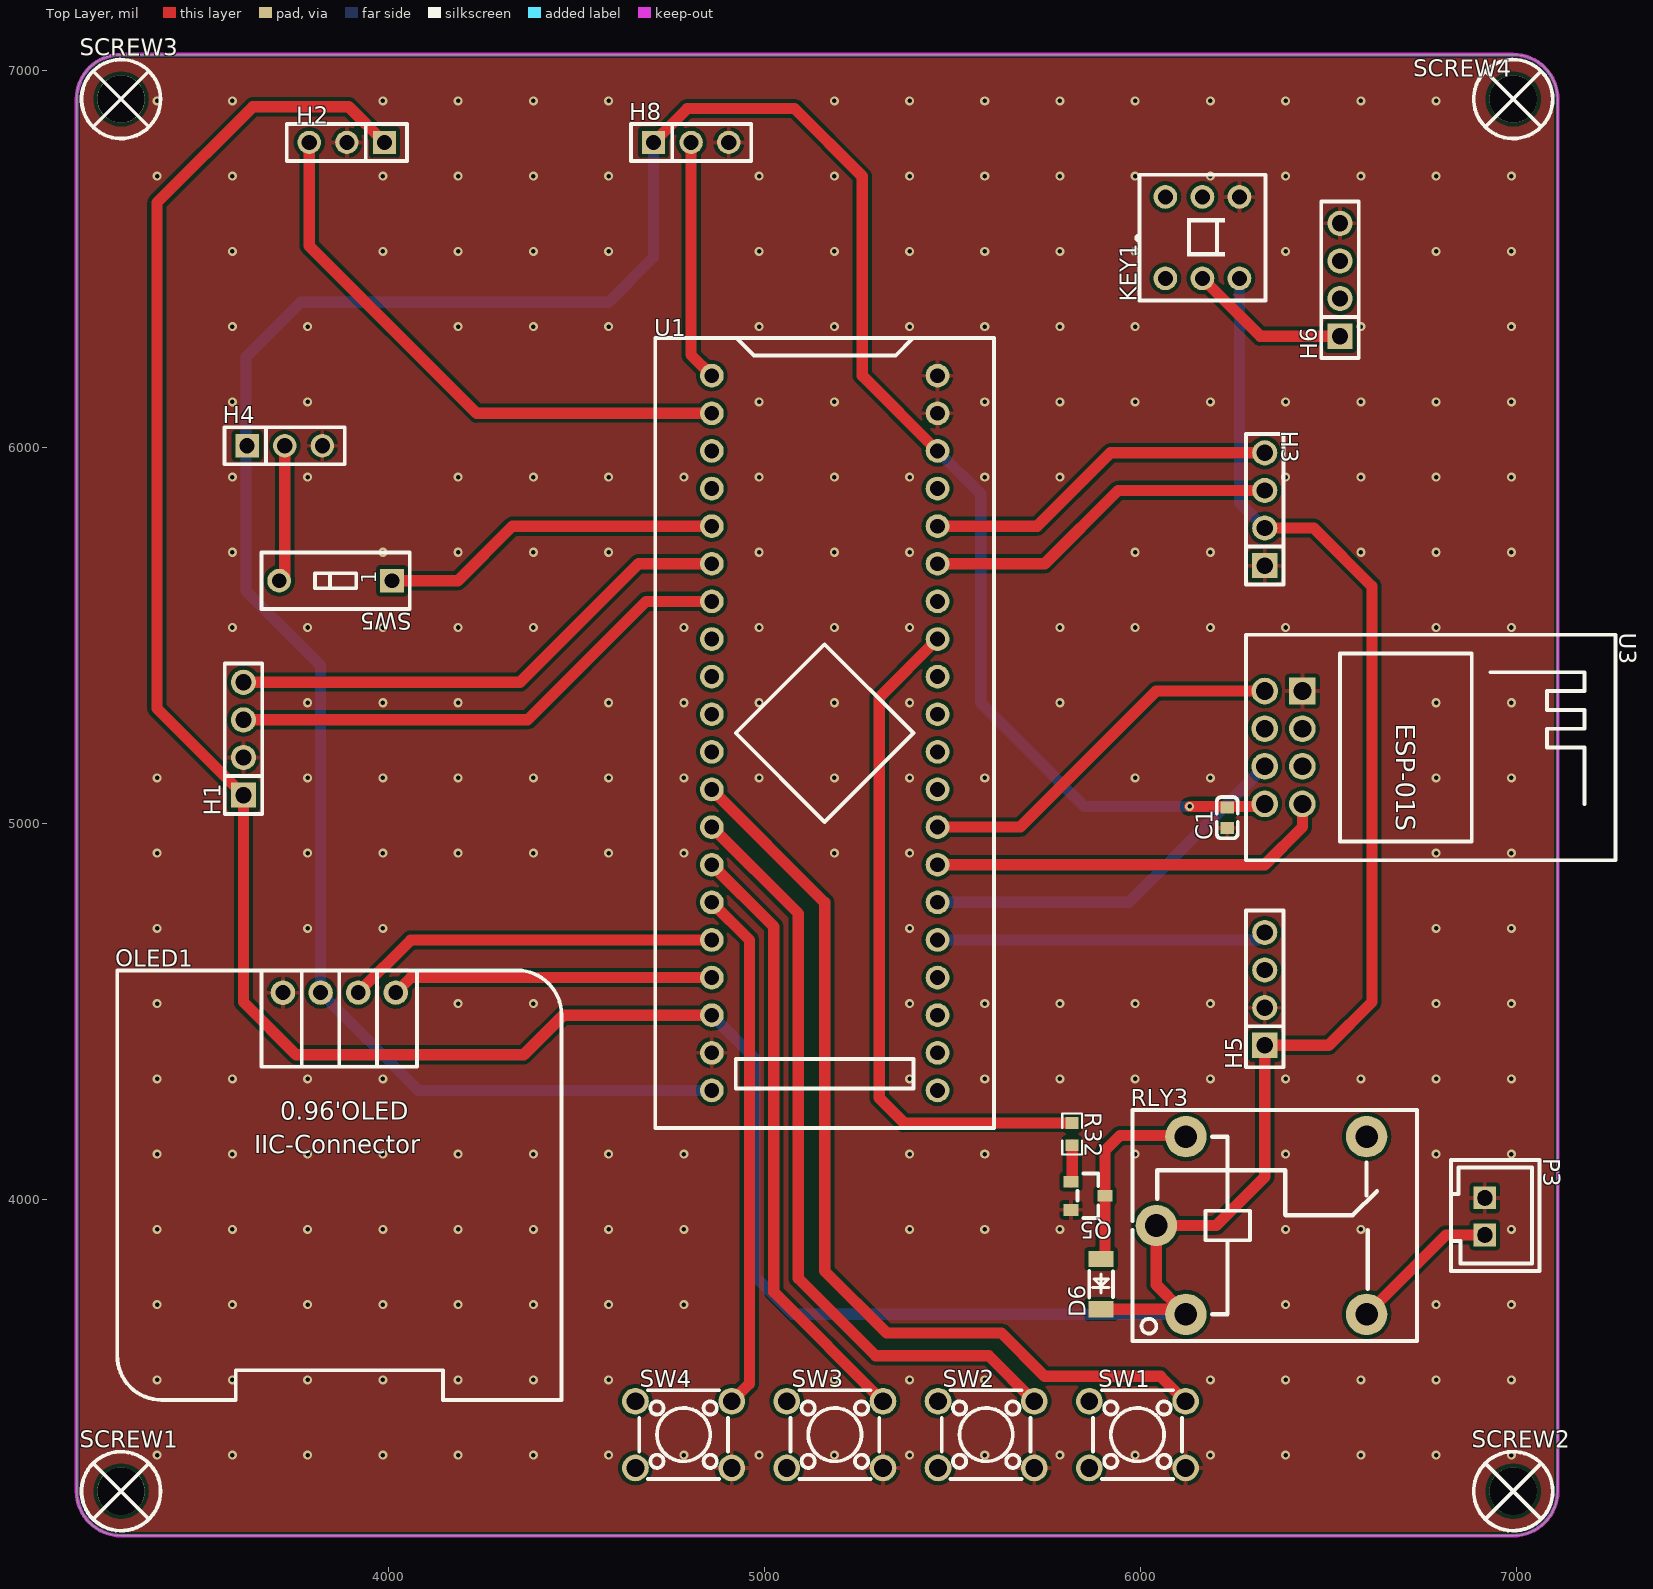
[diagram p0: Top Layer view]
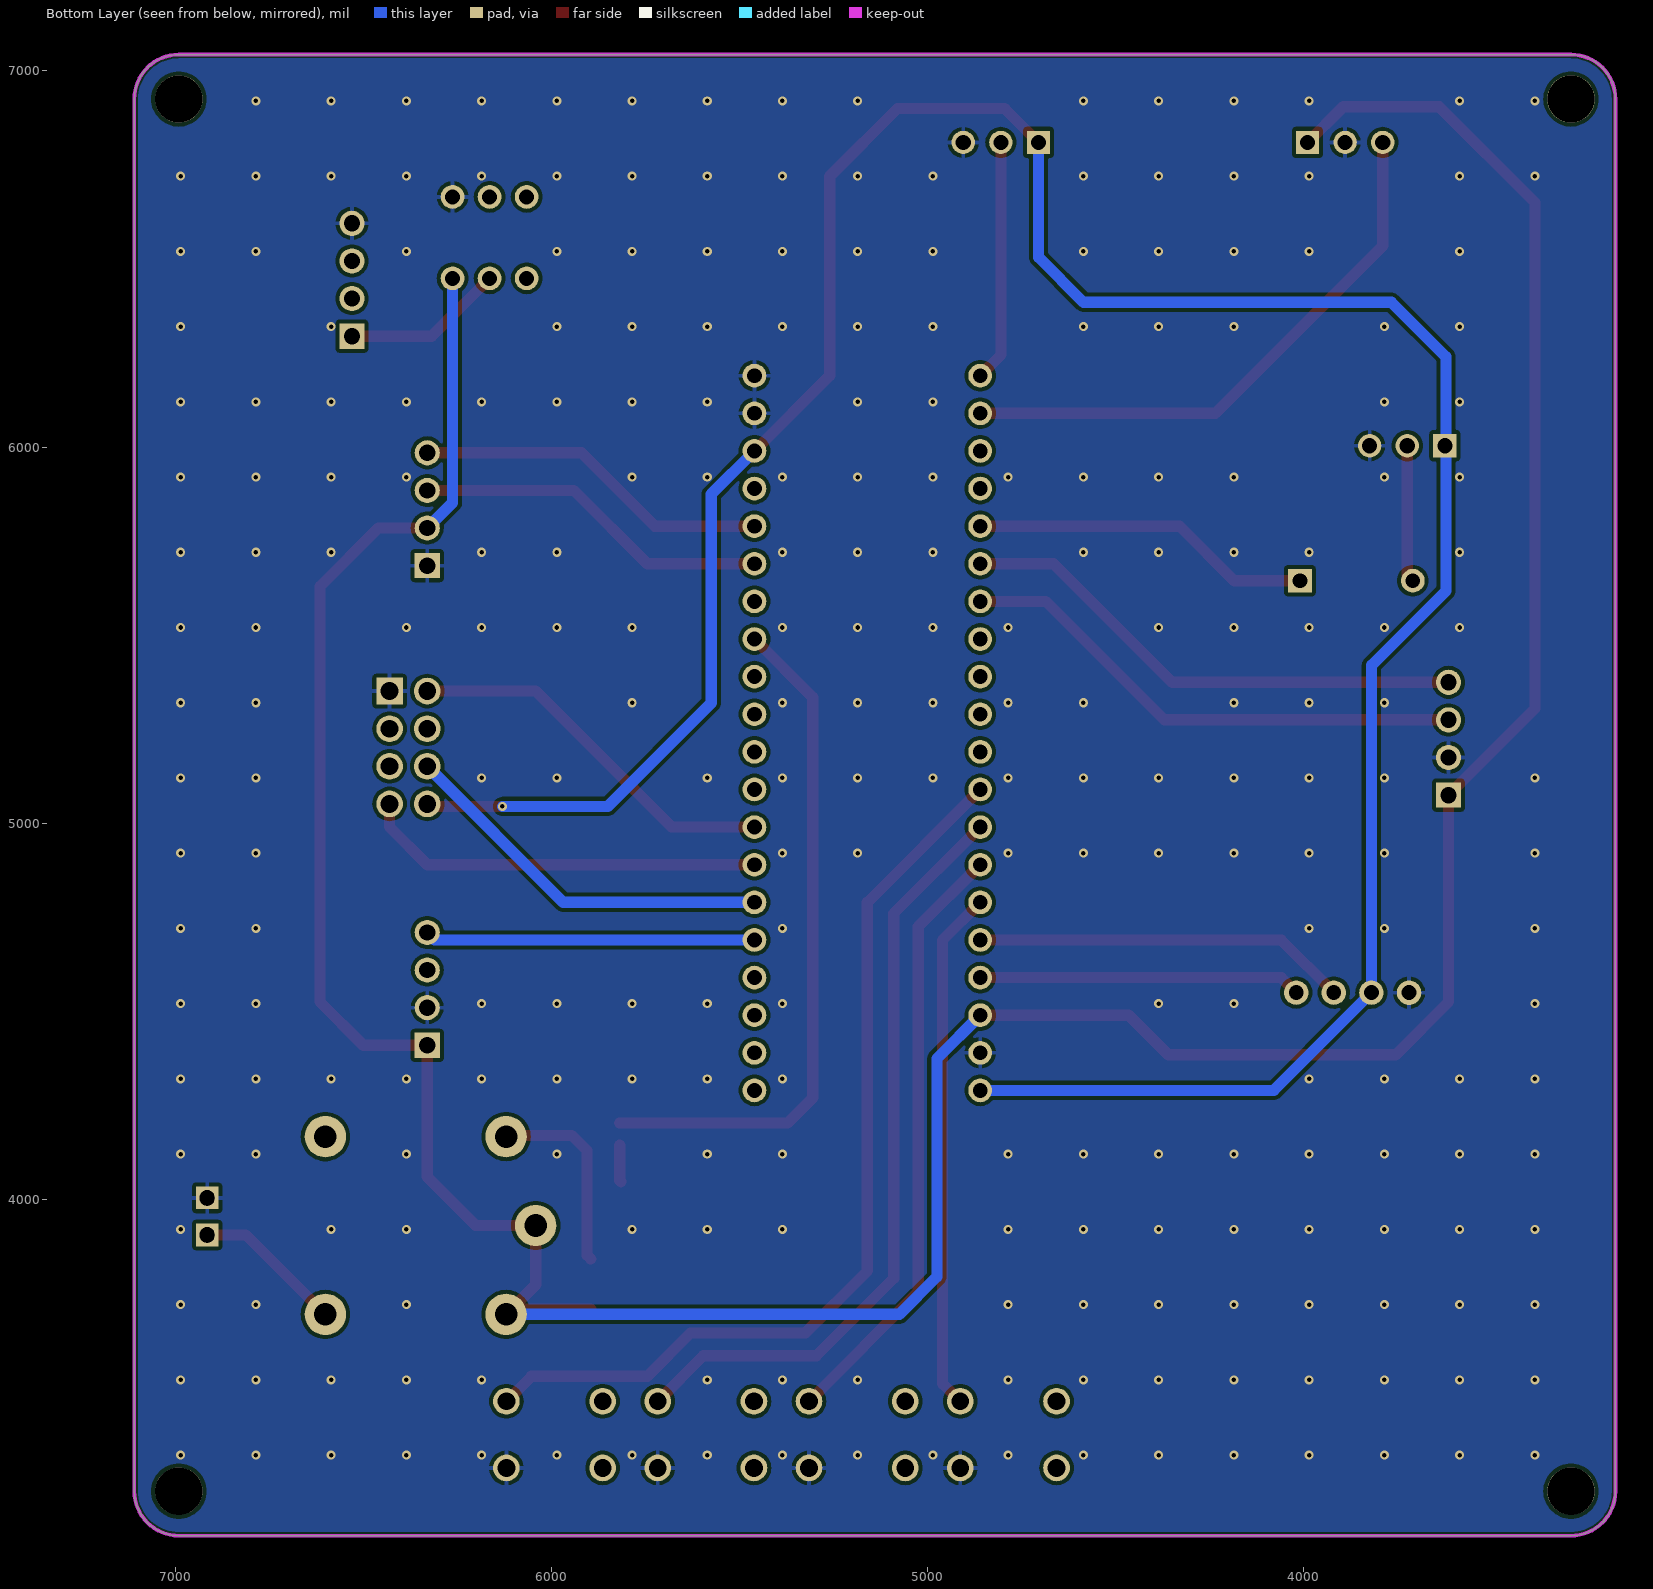
[diagram p1: Bottom Layer view, seen from below]
# Altium PCB MISC75114.pcbdoc
Units mil, origin at the board's own origin, x right, y up, seen from the top; angles counter-clockwise.
Board outline 3937.01 x 3937.01 mil, 2 copper layers (Top Layer, Bottom Layer), stack 62.206 mil thick; 26 components, 42 nets, 121 pads, 255 vias.

## Layer stack, top to bottom
Top Solder Mask Layer: solder mask 0.394, Dk 3.3
Top Layer: signal copper 1.379
Dielectric1: surface 59.449, FR4, Dk 4.5
Bottom Layer: signal copper 1.378
Bottom Solder Mask Layer: solder mask 0.394, Dk 3.3

## Board outline
6990.39,3106.5 ccw(c6990.39,3224.61) 7108.5,3224.61 7108.5,6925.39 ccw(c6990.39,6925.39) 6990.39,7043.5 3289.61,7043.5 ccw(c3289.61,6925.39) 3171.5,6925.39 3171.5,3224.61 ccw(c3289.61,3224.61) 3289.61,3106.5

## Design rules (kind name [scope] priority, off if disabled: settings)
BoardOutlineClearance copperThickness2oz_1 [All] p2 off: genericclearance=7.99 ignorepadtopadclearanceinfootprint=FALSE except(0: Arc-SplitContinuation Track-SplitContinuation SMDPad-SplitContinuation THPad-SplitContinuation Via-SplitContinuation Fill-SplitContinuation Region-SplitContinuation Poly-SplitContinuation Text-SplitContinuation Hole-SplitContinuation; 5.98: Arc-CutoutEdge Track-CutoutEdge SMDPad-CutoutEdge THPad-CutoutEdge Via-CutoutEdge Text-CutoutEdge; 6.89: Hole-OutlineEdge Hole-CutoutEdge; 10: Poly-OutlineEdge Poly-CutoutEdge; 11.81: Arc-OutlineEdge Track-OutlineEdge SMDPad-OutlineEdge THPad-OutlineEdge Via-OutlineEdge Fill-OutlineEdge Region-OutlineEdge Text-OutlineEdge Fill-CutoutEdge Region-CutoutEdge)
BoardOutlineClearance Plane_innerPlane_1 [All] p4 off: genericclearance=4.02 ignorepadtopadclearanceinfootprint=FALSE except(0: Arc-SplitContinuation Track-SplitContinuation SMDPad-SplitContinuation THPad-SplitContinuation Via-SplitContinuation Fill-SplitContinuation Region-SplitContinuation Poly-SplitContinuation Text-SplitContinuation Hole-SplitContinuation; 5.98: Arc-CutoutEdge Track-CutoutEdge SMDPad-CutoutEdge THPad-CutoutEdge Via-CutoutEdge Text-CutoutEdge; 6.89: Hole-OutlineEdge Hole-CutoutEdge; 10: Poly-OutlineEdge Poly-CutoutEdge; 11.81: Arc-OutlineEdge Track-OutlineEdge SMDPad-OutlineEdge THPad-OutlineEdge Via-OutlineEdge Fill-OutlineEdge Region-OutlineEdge Text-OutlineEdge Fill-CutoutEdge Region-CutoutEdge)
BoardOutlineClearance Copper_copperRegion_1 [All] p6 off: genericclearance=4.02 ignorepadtopadclearanceinfootprint=FALSE except(0: Arc-SplitContinuation Track-SplitContinuation SMDPad-SplitContinuation THPad-SplitContinuation Via-SplitContinuation Fill-SplitContinuation Region-SplitContinuation Poly-SplitContinuation Text-SplitContinuation Hole-SplitContinuation; 5.98: Arc-CutoutEdge Track-CutoutEdge SMDPad-CutoutEdge THPad-CutoutEdge Via-CutoutEdge Text-CutoutEdge; 6.89: Hole-OutlineEdge Hole-CutoutEdge; 10: Poly-OutlineEdge Poly-CutoutEdge; 11.81: Arc-OutlineEdge Track-OutlineEdge SMDPad-OutlineEdge THPad-OutlineEdge Via-OutlineEdge Fill-OutlineEdge Region-OutlineEdge Text-OutlineEdge Fill-CutoutEdge Region-CutoutEdge)
BoardOutlineClearance copperThickness1oz_1 [All] p8: genericclearance=4.02 ignorepadtopadclearanceinfootprint=FALSE except(0: Arc-SplitContinuation Track-SplitContinuation SMDPad-SplitContinuation THPad-SplitContinuation Via-SplitContinuation Fill-SplitContinuation Region-SplitContinuation Poly-SplitContinuation Text-SplitContinuation Hole-SplitContinuation; 5.98: Arc-CutoutEdge Track-CutoutEdge SMDPad-CutoutEdge THPad-CutoutEdge Via-CutoutEdge Text-CutoutEdge; 6.89: Hole-OutlineEdge Hole-CutoutEdge; 10: Poly-OutlineEdge Poly-CutoutEdge; 11.81: Arc-OutlineEdge Track-OutlineEdge SMDPad-OutlineEdge THPad-OutlineEdge Via-OutlineEdge Fill-OutlineEdge Region-OutlineEdge Text-OutlineEdge Fill-CutoutEdge Region-CutoutEdge)
Clearance copperThickness2oz [All] p1 off: gap=7.99 ignorepadtopadclearanceinfootprint=FALSE except(5.98: SMDPad-Track SMDPad-SMDPad THPad-Track SMDPad-THPad THPad-THPad Track-Via SMDPad-Via THPad-Via Via-Via Fill-SMDPad Region-SMDPad Fill-THPad Region-THPad Fill-Via Region-Via Fill-Fill Fill-Region Region-Region Arc-Track Arc-SMDPad Arc-THPad Arc-Via Fill-Arc Region-Arc Arc-Arc Text-Track SMDPad-Text Text-THPad Text-Via Fill-Text Region-Text Arc-Text Text-Text; 6.89: Hole-Track Hole-SMDPad Hole-THPad Hole-Via Fill-Hole Region-Hole Hole-Arc Hole-Text; 10: Poly-Track Poly-SMDPad Poly-THPad Poly-Via Poly-Fill Poly-Region Poly-Poly Poly-Arc Poly-Text Poly-Hole; 11.81: Fill-Track Region-Track)
Clearance Plane_innerPlane [All] p3 off: gap=4.02 ignorepadtopadclearanceinfootprint=FALSE except(5.98: SMDPad-Track SMDPad-SMDPad THPad-Track SMDPad-THPad THPad-THPad Track-Via SMDPad-Via THPad-Via Via-Via Fill-SMDPad Region-SMDPad Fill-THPad Region-THPad Fill-Via Region-Via Fill-Fill Fill-Region Region-Region Arc-Track Arc-SMDPad Arc-THPad Arc-Via Fill-Arc Region-Arc Arc-Arc Text-Track SMDPad-Text Text-THPad Text-Via Fill-Text Region-Text Arc-Text Text-Text; 6.89: Hole-Track Hole-SMDPad Hole-THPad Hole-Via Fill-Hole Region-Hole Hole-Arc Hole-Text; 10: Poly-Track Poly-SMDPad Poly-THPad Poly-Via Poly-Fill Poly-Region Poly-Poly Poly-Arc Poly-Text Poly-Hole; 11.81: Fill-Track Region-Track)
Clearance Copper_copperRegion [All] p5 off: gap=4.02 ignorepadtopadclearanceinfootprint=FALSE except(5.98: SMDPad-Track SMDPad-SMDPad THPad-Track SMDPad-THPad THPad-THPad Track-Via SMDPad-Via THPad-Via Via-Via Fill-SMDPad Region-SMDPad Fill-THPad Region-THPad Fill-Via Region-Via Fill-Fill Fill-Region Region-Region Arc-Track Arc-SMDPad Arc-THPad Arc-Via Fill-Arc Region-Arc Arc-Arc Text-Track SMDPad-Text Text-THPad Text-Via Fill-Text Region-Text Arc-Text Text-Text; 6.89: Hole-Track Hole-SMDPad Hole-THPad Hole-Via Fill-Hole Region-Hole Hole-Arc Hole-Text; 10: Poly-Track Poly-SMDPad Poly-THPad Poly-Via Poly-Fill Poly-Region Poly-Poly Poly-Arc Poly-Text Poly-Hole; 11.81: Fill-Track Region-Track)
Clearance copperThickness1oz [All] p7: gap=4.02 ignorepadtopadclearanceinfootprint=FALSE except(5.98: SMDPad-Track SMDPad-SMDPad THPad-Track SMDPad-THPad THPad-THPad Track-Via SMDPad-Via THPad-Via Via-Via Fill-SMDPad Region-SMDPad Fill-THPad Region-THPad Fill-Via Region-Via Fill-Fill Fill-Region Region-Region Arc-Track Arc-SMDPad Arc-THPad Arc-Via Fill-Arc Region-Arc Arc-Arc Text-Track SMDPad-Text Text-THPad Text-Via Fill-Text Region-Text Arc-Text Text-Text; 6.89: Hole-Track Hole-SMDPad Hole-THPad Hole-Via Fill-Hole Region-Hole Hole-Arc Hole-Text; 10: Poly-Track Poly-SMDPad Poly-THPad Poly-Via Poly-Fill Poly-Region Poly-Poly Poly-Arc Poly-Text Poly-Hole; 11.81: Fill-Track Region-Track)
DiffPairsRouting differentialPair [All] p1: maxlimit=6 minlimit=6 mostfreqgap=6 toplayer_minwidth=5 toplayer_prefwidth=10 toplayer_maxwidth=100 toplayer_mingap=6 toplayer_prefgap=6 toplayer_maxgap=6 bottomlayer_minwidth=5 bottomlayer_prefwidth=10 bottomlayer_maxwidth=100 bottomlayer_mingap=6 bottomlayer_prefgap=6 bottomlayer_maxgap=6 maxuncoupledlength=10
HoleToHoleClearance otherClearance [All] p1: gap=11.81 allowstackedmicrovias=TRUE
Length netLength [All] p1: minlimit=0 maxlimit=0
PasteMaskExpansion pasteMaskExpansion [All] p1: expansion=0
PlaneConnect innerPlane [All] p1: planeconnectstyle=Relief reliefexpansion=20 reliefentries=4 reliefconductorwidth=10 reliefairgap=10
PolygonConnect copperRegion [All] p1: connectstyle=Relief reliefconductorwidth=10 reliefentries=4 polygonreliefangle="90 Angle" airgapwidth=10 via.connectstyle=Relief via.reliefconductorwidth=10 via.reliefentries=4 via.polygonreliefangle="90 Angle" via.airgapwidth=10
RoutingVias viaSize [All] p1: holewidth=12.01 width=24.02 viastyle="Through Hole" minholewidth=11.81 minwidth=19.68 maxholewidth=248.03 maxwidth=393.7
SolderMaskExpansion solderMaskExpansion [IsVia] p1: expansion=-1000 istentingtop=TRUE
SolderMaskExpansion solderMaskExpansion [All] p2: expansion=2.01 istentingtop=FALSE
Width copperThickness2oz_2 [All] p1 off: maxlimit=100 minlimit=8 preferedwidth=10
Width copperThickness1oz_2 [All] p2: maxlimit=100 minlimit=5 preferedwidth=30

## Components (designator, comment, footprint, x,y, rotation, side; value= is the part's Value field where it differs from the comment)
C1 "1uF" C0603 6230,5015 r90 top
D6 "LL4148" LL-34_L3.5-W1.5-RD 5895,3775 r90 top
H1 "" HDR-TH_4P-P2.54-V-M 3615,5225 r90 top
H2 "" HDR-TH_3P-P2.54-V-F 3890,6810 r180 top
H3 "" HDR-TH_4P-P2.54-V-M 6329.9,5835 r90 top
H4 "" HDR-TH_3P-P2.54-V-F 3724.74,6003.84 r0 top
H5 "" HDR-TH_4P-P2.54-V-F 6329.9,4560 r90 top
H6 "" HDR-TH_4P-P2.54-V-F 6530,6445 r90 top
H8 "" HDR-TH_3P-P2.54-V-F 4805,6810 r0 top
KEY1 "Non-latching switch 8.5×8.5 silent" SW-TH_6P-L8.5-W8.5-P2.54 6164.22,6556.9 r0 top
OLED1 "" 0.96OLED_4P 3870,4550 r0 top
P3 "XH2.54 through-hole socket-2P" CONN-TH_XH2.54-2P 6915,3954.99 r270 top
Q5 "" S8050_SOT-23 5860,4015 r180 top
R32 "1k" R0603 5817.82,4173.92 r270 top
RLY3 "SRD-05VDC-SL-C" RELAY-TH_SRD-XXVDC-XL-C 6321.15,3930.95 r0 top
SCREW1 "" M3螺丝 3289.61,3224.61 r0 top
SCREW2 "" M3螺丝 6990.39,3224.61 r0 top
SCREW3 "" M3螺丝 3289.61,6925.39 r0 top
SCREW4 "" M3螺丝 6990.39,6925.39 r0 top
SW1 "" SW-TH_4P-L6.0-W6.0-P4.50-LS6.5 5991.57,3375 r180 top
SW2 "" SW-TH_4P-L6.0-W6.0-P4.50-LS6.5 5589.38,3375 r180 top
SW3 "" SW-TH_4P-L6.0-W6.0-P4.50-LS6.5 5187.19,3375 r180 top
SW4 "" SW-TH_4P-L6.0-W6.0-P4.50-LS6.5 4785,3375 r180 top
SW5 "NDS-01V" SW-TH_2P-L3.9-W9.9-P2.54-LS7.6 3860,5645 r180 top
U1 "STM32F103C8T6-Card" CONN-TH_L53.3-W22.9_STM32F103C8T6-CARD 5160,5240 r270 top
U3 "ESP-01S" WIFIM-TH_ESP-01S 6380,5201.63 r270 top

## Footprints (in the part's own frame and the unit in brackets; to place one, negate y for a bottom-side part, rotate by r counter-clockwise, add the part's x,y. Pads: shape width x height; smd on the part's side, far side on the other; paste and mask are expansions set on the pad)
0.96OLED_4P [mm]
  round 1.65 hole 1 copper offset 0,0: 1(-3.81,-0.001) 2(-1.27,0.002) 3(1.27,0.002) 4(3.81,0.002)
  silkscreen extent -15,-27.5 15,1.5
C0603 [mm]
  rect 0.8x0.9 smd: 1(-0.7,0) 2(0.7,0)
  silkscreen extent -1.39,-0.71 1.39,0.71
CONN-TH_L53.3-W22.9_STM32F103C8T6-CARD [mm]
  round 1.6 hole 1: 1(-24.13,-7.62) 2(-21.59,-7.62) 3(-19.05,-7.62) 4(-16.51,-7.62) 5(-13.97,-7.62) 6(-11.43,-7.62) 7(-8.89,-7.62) 8(-6.35,-7.62) 9(-3.81,-7.62) 10(-1.27,-7.62) 11(1.27,-7.62) 12(3.81,-7.62) 13(6.35,-7.62) 14(8.89,-7.62) 15(11.43,-7.62) 16(13.97,-7.62) 17(16.51,-7.62) 18(19.05,-7.62) 19(21.59,-7.62) 20(24.13,-7.62) 21(24.13,7.62) 22(21.59,7.62) 23(19.05,7.62) 24(16.51,7.62) 25(13.97,7.62) 26(11.43,7.62) 27(8.89,7.62) 28(6.35,7.62) 29(3.81,7.62) 30(1.27,7.62) 31(-1.27,7.62) 32(-3.81,7.62) 33(-6.35,7.62) 34(-8.89,7.62) 35(-11.43,7.62) 36(-13.97,7.62) 37(-16.51,7.62) 38(-19.05,7.62) 39(-21.59,7.62) 40(-24.13,7.62)
  silkscreen extent -26.67,-11.43 26.67,11.43
CONN-TH_XH2.54-2P [mil]
  rect 60x60 hole 39.37 slot 41.34 at 0 deg paste+0 mask+1.97: 1(-49.22,0) 2(49.21,0)
  silkscreen extent -150,-90 145,145
HDR-TH_3P-P2.54-V-F [mil]
  rect 62x62 hole 40.16: 1(-100,0)
  round 62 hole 40.16: 2(0,0) 3(100,0)
  silkscreen extent -160,-49 160,49
HDR-TH_4P-P2.54-V-F [mm]
  rect 1.7x1.7 hole 1.1: 1(-3.81,0)
  round 1.7 hole 1.1: 2(-1.27,0) 3(1.27,0) 4(3.81,0)
  silkscreen extent -5.29,-1.27 5.29,1.27
HDR-TH_4P-P2.54-V-M [mm]
  rect 1.7x1.7 hole 1.1: 1(-3.81,0)
  round 1.7 hole 1.1: 2(-1.27,0) 3(1.27,0) 4(3.81,0)
  silkscreen extent -5.08,-1.27 5.08,1.27
LL-34_L3.5-W1.5-RD [mm]
  rect 1.1x1.7 smd paste+0 mask+0.051: 1(-1.7,0) 2(1.7,0)
  silkscreen extent -0.9,-0.8 0.9,0.8
M3螺丝 [mil]
  round 126 hole 126 paste+0 mask+4: 1(0,0)
  silkscreen extent -105,-105 105,105
R0603 [mil]
  rect 31.75x34.02 smd paste-3937.01 mask+2: 1(-29.66,0) 2(29.66,0)
  silkscreen extent -55,-26 55,26
RELAY-TH_SRD-XXVDC-XL-C [mil]
  round 110 hole 60: 1(-200.79,-236.22) 2(279.52,-236.2) 3(279.53,236.2) 4(-200.79,236.22) 5(-279.53,0)
  silkscreen extent -342,-307 413,307
S8050_SOT-23 [mm]
  rect 1x0.8 smd paste+0 mask+0.051: 1(1.15,-0.823) 2(1.15,1.077) 3(-1.15,0.127)
  silkscreen extent -0.7,-1.37 0.7,1.63
SW-TH_2P-L3.9-W9.9-P2.54-LS7.6 [mm]
  rect 1.6x1.6 hole 1 paste+0 mask+0.05: 1(-3.81,0)
  round 1.6 hole 1 paste+0 mask+0.05: 2(3.81,0)
  silkscreen extent -5,-1.91 5,1.91
SW-TH_4P-L6.0-W6.0-P4.50-LS6.5 [mm]
  round 1.8 hole 1.2: 1(-3.25,2.25) 2(3.25,2.25) 3(-3.25,-2.25) 4(3.25,-2.25)
  silkscreen extent -3,-3 3,3
SW-TH_6P-L8.5-W8.5-P2.54 [mm]
  round 1.6 hole 1: 1(-2.5,-2.75) 2(0,-2.75) 3(2.5,-2.75) 4(-2.5,2.75) 5(0,2.75) 6(2.5,2.75)
  silkscreen extent -4.47,-4.25 4.25,4.25
WIFIM-TH_ESP-01S [mm]
  rect 1.8x1.8 hole 1.2: 1(-3.81,1.27)
  round 1.8 hole 1.2: 2(-1.27,1.27) 3(1.27,1.27) 4(3.81,1.27) 5(3.81,-1.27) 6(1.27,-1.27) 7(-1.27,-1.27) 8(-3.81,-1.27)
  silkscreen extent -7.62,-2.54 7.62,22.4

## Via types
v1: diameter 24.02, hole 12, Top Layer to Bottom Layer, 255 vias

## Nets (pads, with @x,y where several pads share a name; then routed paths per layer and width w, separated by ;. In a path a pad name is that pad's centre, name@x,y a point inside that pad or via, vN(x,y) a via of type N, cw(c..) or ccw(c..) an arc to the next point about the centre after c; other vN are vias at no path point)
$1N18282: H6.1 KEY1.2 | length 429.4
  Top Layer w30: KEY1.2 6317.84,6295 H6.1
$1N18356: Q5.1 R32.2 | length 98.1
  Top Layer w30: Q5.1 5817.82,4050.5 R32.2
$1N18358: D6.2 Q5.3 RLY3.4 | length 525.3
  Top Layer w30: D6.2 5905.28,3852.21 Q5.3 5905.28,4130.28 5945,4170 6117.53,4170 RLY3.4
$1N18360: P3.2 RLY3.2 | length 401.7
  Top Layer w30: RLY3.2 6811.7,3905.78 P3.2
$1N18374: H4.2 SW5.2 | length 364.9
  Top Layer w30: SW5.2 3724.74,5659.74 H4.2
+5V: D6.1 H1.1 H2.1 H3.2 H5.1 KEY1.3 RLY3.1 RLY3.5 U1.18 | length 9878.6
  Top Layer w30: H2.1 3895,6905 3640,6905 3385,6650 3385,5305 H1.1 3615,4525 3755,4385 4360,4385 4465,4490 U1.18 ; D6.1 6107.02,3708.07 6041.62,3773.47 RLY3.5 6200.95,3930.95 6329.9,4059.9 H5.1 6500,4410 6615,4525 6615,5630 6460,5785 H3.2
  Bottom Layer w30: U1.18 4975,4375 4975,3795 5075.27,3694.73 RLY3.1 ; KEY1.3 6262.64,5852.26 H3.2
GND: C1.1 H1.2 H2.2 H3.1 H4.3 H5.2 H6.4 H8.3 KEY1.6 OLED1.1 P3.1 Q5.2 SW1.1 SW2.1 SW3.1 SW4.1 U1.19 U1.39 U1.40 U3.1
  other v1: 3385.6,3320.6 3585.6,3320.6 3785.6,3320.6 3985.6,3320.6 4185.6,3320.6 4385.6,3320.6 4585.6,3320.6 4785.6,3320.6 4985.6,3320.6 5185.6,3320.6 5385.6,3320.6 5585.6,3320.6 5785.6,3320.6 5985.6,3320.6 6185.6,3320.6 6385.6,3320.6 6585.6,3320.6 6785.6,3320.6 6985.6,3320.6 3385.6,3520.6 3585.6,3520.6 3785.6,3520.6 3985.6,3520.6 4185.6,3520.6 4385.6,3520.6 4585.6,3520.6 4785.6,3520.6 5185.6,3520.6 5385.6,3520.6 5585.6,3520.6 6185.6,3520.6 6385.6,3520.6 6585.6,3520.6 6785.6,3520.6 6985.6,3520.6 3385.6,3720.6 3585.6,3720.6 3785.6,3720.6 3985.6,3720.6 4185.6,3720.6 4385.6,3720.6 4585.6,3720.6 4785.6,3720.6 6385.6,3720.6 6785.6,3720.6 6985.6,3720.6 3385.6,3920.6 3585.6,3920.6 3785.6,3920.6 3985.6,3920.6 4185.6,3920.6 4385.6,3920.6 4585.6,3920.6 4785.6,3920.6 5385.6,3920.6 5585.6,3920.6 5785.6,3920.6 6385.6,3920.6 6585.6,3920.6 6985.6,3920.6 3385.6,4120.6 3585.6,4120.6 3785.6,4120.6 3985.6,4120.6 4185.6,4120.6 4385.6,4120.6 4585.6,4120.6 4785.6,4120.6 5385.6,4120.6 5585.6,4120.6 5985.6,4120.6 6385.6,4120.6 6785.6,4120.6 6985.6,4120.6 3385.6,4320.6 3585.6,4320.6 3785.6,4320.6 3985.6,4320.6 5385.6,4320.6 5585.6,4320.6 5785.6,4320.6 5985.6,4320.6 6185.6,4320.6 6385.6,4320.6 6585.6,4320.6 6785.6,4320.6 6985.6,4320.6 3385.6,4520.6 4185.6,4520.6 4385.6,4520.6 5385.6,4520.6 5585.6,4520.6 5785.6,4520.6 5985.6,4520.6 6185.6,4520.6 6785.6,4520.6 6985.6,4520.6 3385.6,4720.6 3785.6,4720.6 3985.6,4720.6 5385.6,4720.6 6785.6,4720.6 6985.6,4720.6 3385.6,4920.6 3785.6,4920.6 3985.6,4920.6 4185.6,4920.6 4385.6,4920.6 4585.6,4920.6 4785.6,4920.6 5185.6,4920.6 5385.6,4920.6 6785.6,4920.6 6985.6,4920.6 3385.6,5120.6 3785.6,5120.6 3985.6,5120.6 4185.6,5120.6 4385.6,5120.6 4585.6,5120.6 4785.6,5120.6 4985.6,5120.6 5185.6,5120.6 5385.6,5120.6 5585.6,5120.6 5985.6,5120.6 6185.6,5120.6 6785.6,5120.6 6985.6,5120.6 3785.6,5320.6 3985.6,5320.6 4185.6,5320.6 4585.6,5320.6 4785.6,5320.6 4985.6,5320.6 5185.6,5320.6 5385.6,5320.6 5785.6,5320.6 6785.6,5320.6 6985.6,5320.6 3585.6,5520.6 3785.6,5520.6 3985.6,5520.6 4185.6,5520.6 4385.6,5520.6 4785.6,5520.6 4985.6,5520.6 5185.6,5520.6 5385.6,5520.6 5785.6,5520.6 5985.6,5520.6 6185.6,5520.6 6385.6,5520.6 6785.6,5520.6 6985.6,5520.6 3585.6,5720.6 3985.6,5720.6 4185.6,5720.6 4385.6,5720.6 4585.6,5720.6 4985.6,5720.6 5185.6,5720.6 5385.6,5720.6 5985.6,5720.6 6185.6,5720.6 6585.6,5720.6 6785.6,5720.6 6985.6,5720.6 3585.6,5920.6 3785.6,5920.6 4185.6,5920.6 4385.6,5920.6 4585.6,5920.6 4785.6,5920.6 4985.6,5920.6 5185.6,5920.6 5385.6,5920.6 5585.6,5920.6 5785.6,5920.6 6385.6,5920.6 6585.6,5920.6 6785.6,5920.6 6985.6,5920.6 3585.6,6120.6 3785.6,6120.6 4985.6,6120.6 5185.6,6120.6 5585.6,6120.6 5785.6,6120.6 5985.6,6120.6 6185.6,6120.6 6385.6,6120.6 6585.6,6120.6 6785.6,6120.6 6985.6,6120.6 3585.6,6320.6 3785.6,6320.6 4185.6,6320.6 4385.6,6320.6 4585.6,6320.6 4985.6,6320.6 5185.6,6320.6 5385.6,6320.6 5585.6,6320.6 5785.6,6320.6 5985.6,6320.6 6585.6,6320.6 6985.6,6320.6 3585.6,6520.6 3985.6,6520.6 4185.6,6520.6 4385.6,6520.6 4585.6,6520.6 4985.6,6520.6 5185.6,6520.6 5385.6,6520.6 5585.6,6520.6 5785.6,6520.6 5985.6,6520.6 6385.6,6520.6 6785.6,6520.6 6985.6,6520.6 3385.6,6720.6 3585.6,6720.6 3985.6,6720.6 4185.6,6720.6 4385.6,6720.6 4585.6,6720.6 4985.6,6720.6 5185.6,6720.6 5385.6,6720.6 5585.6,6720.6 5785.6,6720.6 5985.6,6720.6 6185.6,6720.6 6385.6,6720.6 6585.6,6720.6 6785.6,6720.6 6985.6,6720.6 3385.6,6920.6 3585.6,6920.6 3985.6,6920.6 4185.6,6920.6 4385.6,6920.6 4585.6,6920.6 5185.6,6920.6 5385.6,6920.6 5585.6,6920.6 5785.6,6920.6 5985.6,6920.6 6185.6,6920.6 6385.6,6920.6 6585.6,6920.6 6785.6,6920.6
NRST: U1.37
PA0: H5.4 U1.25 | length 878.2
  Bottom Layer w30: U1.25 6309.9,4690 H5.4
PA1: U1.26 U3.6 | length 1019.8
  Bottom Layer w30: U1.26 5968.36,4790 U3.6
PA2: U1.27 U3.4 | length 1073.1
  Top Layer w30: U1.27 6330,4890 6430,4990 U3.4
PA3: U1.28 U3.8 | length 1019.8
  Top Layer w30: U1.28 5680,4990 6041.63,5351.63 U3.8
PA4: U1.29
PA5: U1.30
PA6: U1.31
PA7: U1.32
PA8: SW5.1 U1.5 | length 910.1
  Top Layer w30: SW5.1 4185,5645 4330,5790 U1.5
PA9: H1.4 U1.6 | length 1375.5
  Top Layer w30: H1.4 4350,5375 4665,5690 U1.6
PA10: H1.3 U1.7 | length 1375.5
  Top Layer w30: H1.3 4370,5275 4685,5590 U1.7
PA11: U1.8
PA12: U1.9
PA15: U1.10
PB0: R32.1 U1.33 | length 1824.5
  Top Layer w30: U1.33 5305,5335 5305,4270 5371.42,4203.58 R32.1
PB1: U1.34
PB3: U1.11
PB4: SW1.3 U1.12 | length 2507.3
  Top Layer w30: U1.12 5160,4790 5160,3810 5325,3645 5630,3645 5745,3530 6053.1,3530 SW1.3
PB5: SW2.3 U1.13 | length 2057.8
  Top Layer w30: U1.13 5090,4760 5090,3790 5295,3585 5595.91,3585 SW2.3
PB6: SW3.3 U1.14 | length 1614.9
  Top Layer w30: U1.14 5025,4725 5025,3753.72 SW3.3
PB7: SW4.3 U1.15 | length 1387.3
  Top Layer w30: U1.15 4960,4690 4960,3510.63 SW4.3
PB8: OLED1.3 U1.16 | length 998
  Top Layer w30: OLED1.3@3920,4550.05 4059.95,4690 U1.16
PB9: OLED1.4 U1.17 | length 856.5
  Top Layer w30: OLED1.4@4020,4550.05 4059.95,4590 U1.17
PB10: H3.3 U1.35 | length 950.7
  Top Layer w30: U1.35 5745,5690 5940,5885 H3.3
PB11: H3.4 U1.36 | length 950.7
  Top Layer w30: U1.36 5725,5790 5920,5985 H3.4
PB12: H8.2 U1.1 | length 642.8
  Top Layer w30: H8.2 4805,6245 U1.1
PB13: H2.3 U1.2 | length 1529.3
  Top Layer w30: H2.3 3790,6535 4235,6090 U1.2
PB14: U1.3
PB15: U1.4
PC13: U1.22
PC14: U1.23
PC15: U1.24
VBAT: U1.21
VCC: C1.2 H4.1 H8.1 OLED1.2 U1.20 U1.38 U3.5 | length 7486.6
  Top Layer w30: H8.1 4795,6900 5080,6900 5260,6720 5260,6190 U1.38 ; v1(6130,5045) 6323.37,5045 U3.5
  Bottom Layer w30: H8.1 4705,6505 4585,6385 3766.89,6385 3621.89,6240 3621.89,5618.11 3820,5420 3820,4550.05 4080.05,4290 U1.20 ; U1.38 5575,5875 5575,5320 5850,5045 v1(6130,5045)
pads on no net: H5.3 H6.2 H6.3 KEY1.1 KEY1.4 KEY1.5 RLY3.3 SCREW1.1 SCREW2.1 SCREW3.1 SCREW4.1 SW1.2 SW1.4 SW2.2 SW2.4 SW3.2 SW3.4 SW4.2 SW4.4 U3.2 U3.3 U3.7

## Polygon pours and split planes (outlines as drawn)
GND on Bottom Layer (solid, remove dead copper, pour order 2): 3100,7165 3100,3000 7275,3000 7275,7165
GND on Top Layer (solid, remove dead copper, pour order 0): 3000,7145 3000,3075 7385,3075 7385,7145

## Keep-outs
Board Outline Layer:
  the board outline again, w10